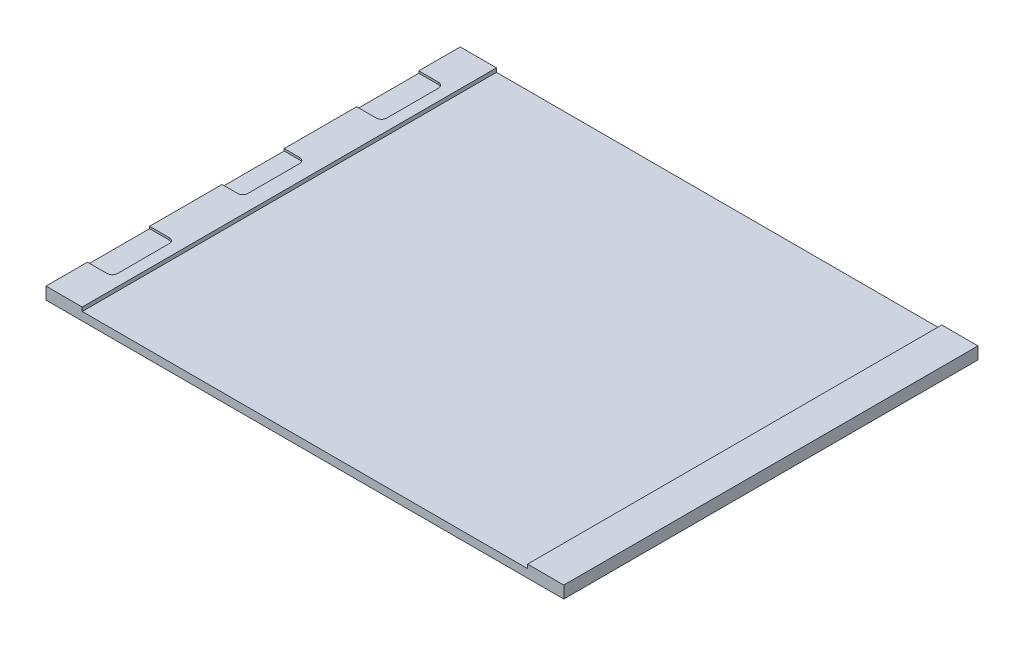
from build123d import *

# Parameters (mm, degrees)
SKETCH1_W           = 500
SKETCH1_H           = 24
BOSS_EXTRUDE1_DEPTH = 400
SKETCH2_W           = 430
SKETCH2_H           = 8
CUT_EXTRUDE1_DEPTH  = 641.762046317
SKETCH3_W           = 544.957019416
SKETCH3_H           = 0.5
CUT_EXTRUDE2_DEPTH  = 641.762046317
SKETCH12_W          = 569.007892772
SKETCH12_H          = 39.328779912
CUT_EXTRUDE3_DEPTH  = 641.762046317
SKETCH16_W          = 24
SKETCH16_H          = 60
SKETCH16_W_2        = 20
CUT_EXTRUDE4_DEPTH  = 2
FILLET1_R           = 5


with BuildPart() as part:
    # Sketch1 → Boss-Extrude1 (new body)
    with BuildSketch(Plane.XY):
        with Locations((250, 12)):
            Rectangle(SKETCH1_W, SKETCH1_H)
    extrude(amount=-BOSS_EXTRUDE1_DEPTH)

    # Sketch2 → Cut-Extrude1 (cut, through all)
    with BuildSketch(Plane.XY):
        with Locations((250, 12)):
            Rectangle(SKETCH2_W, SKETCH2_H)
    extrude(amount=-CUT_EXTRUDE1_DEPTH, mode=Mode.SUBTRACT)

    # Sketch3 → Cut-Extrude2 (cut, through all)
    with BuildSketch(Plane.XY):
        with Locations((250, 12)):
            Rectangle(SKETCH3_W, SKETCH3_H)
    extrude(amount=-CUT_EXTRUDE2_DEPTH, mode=Mode.SUBTRACT)


with BuildPart() as cut_extrude2_piece_1:
    # of the separate pieces the step leaves, piece 1, a body of its own (cut_extrude2_pieces)
    add(part.part.solids().sort_by_distance((0, 0, 0))[0])

    # Sketch16 → Cut-Extrude4 (cut)
    with BuildSketch(Plane(origin=(0, 11.75, 0), x_dir=(1, 0, 0), z_dir=(0, 1, 0))):
        with Locations((12, 330)):
            Rectangle(SKETCH16_W, SKETCH16_H)
        with Locations((12, 70)):
            Rectangle(SKETCH16_W, SKETCH16_H)
        with Locations((10, 200)):
            Rectangle(SKETCH16_W_2, SKETCH16_H)
    extrude(amount=-CUT_EXTRUDE4_DEPTH, mode=Mode.SUBTRACT)

    # Fillet1
    fillet1_edges = [cut_extrude2_piece_1.edges().sort_by_distance(p)[0] for p in [
        (24, 10.75, -360),
        (24, 10.75, -300),
        (24, 10.75, -40),
        (24, 10.75, -100),
        (20, 10.75, -230),
        (20, 10.75, -170),
    ]]
    fillet(fillet1_edges, radius=FILLET1_R)


with BuildPart() as cut_extrude2_piece_2:
    # of the separate pieces the step leaves, piece 2, a body of its own (cut_extrude2_pieces)
    add(part.part.solids().sort_by_distance((0, 24, 0))[0])

    # Sketch12 → Cut-Extrude3 (cut, through all)
    with BuildSketch(Plane.XY):
        with Locations((265.175540793, 31.664389956)):
            Rectangle(SKETCH12_W, SKETCH12_H)
    extrude(amount=-CUT_EXTRUDE3_DEPTH, mode=Mode.SUBTRACT)


solid = cut_extrude2_piece_1.part
